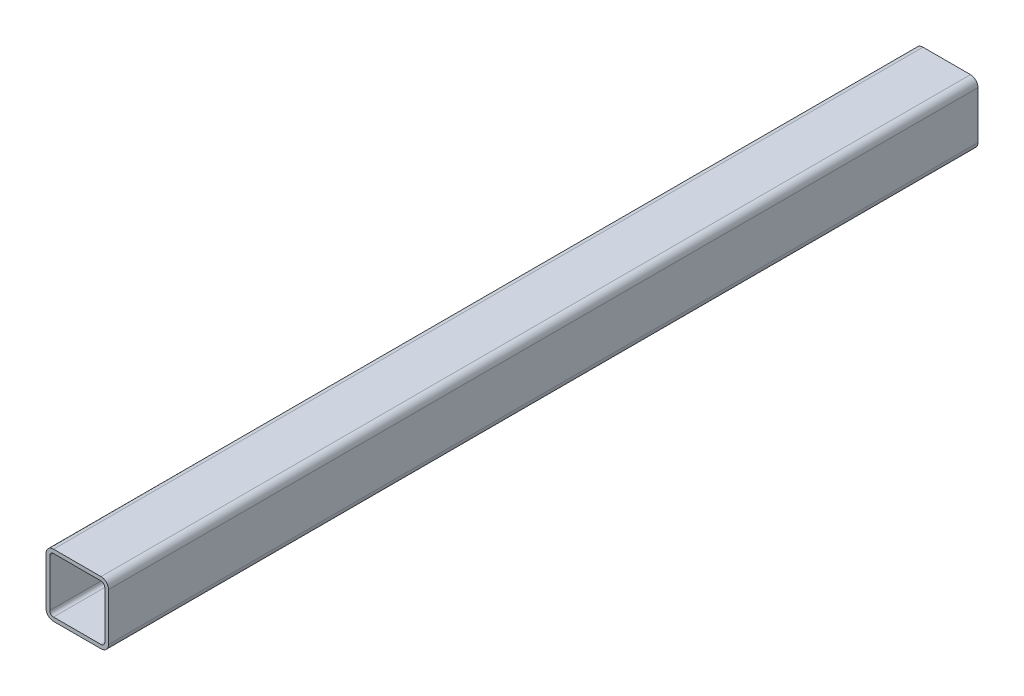
from build123d import *

# Parameters (mm, degrees)
GB_6728_1986_050_X_50_X_3_1_DEPTH = 695


with BuildPart() as part:
    # Sketch1 → Gb／6728-1986方形空心型钢 050 X 50 X 3(1) (new body)
    with BuildSketch(Plane.YX.offset(-347.5)):
        with BuildLine():
            Line((-19, -25), (19, -25))
            ThreePointArc((19, -25), (23.242640687, -23.242640687), (25, -19))
            Line((25, -19), (25, 19))
            ThreePointArc((25, 19), (23.242640687, 23.242640687), (19, 25))
            Line((19, 25), (-19, 25))
            ThreePointArc((-19, 25), (-23.242640687, 23.242640687), (-25, 19))
            Line((-25, 19), (-25, -19))
            ThreePointArc((-25, -19), (-23.242640687, -23.242640687), (-19, -25))
        make_face()
        with BuildLine():
            Line((-19, -22), (19, -22))
            ThreePointArc((19, -22), (21.121320344, -21.121320344), (22, -19))
            Line((22, -19), (22, 19))
            ThreePointArc((22, 19), (21.121320344, 21.121320344), (19, 22))
            Line((19, 22), (-19, 22))
            ThreePointArc((-19, 22), (-21.121320344, 21.121320344), (-22, 19))
            Line((-22, 19), (-22, -19))
            ThreePointArc((-22, -19), (-21.121320344, -21.121320344), (-19, -22))
        make_face(mode=Mode.SUBTRACT)
    extrude(amount=GB_6728_1986_050_X_50_X_3_1_DEPTH)


solid = part.part
